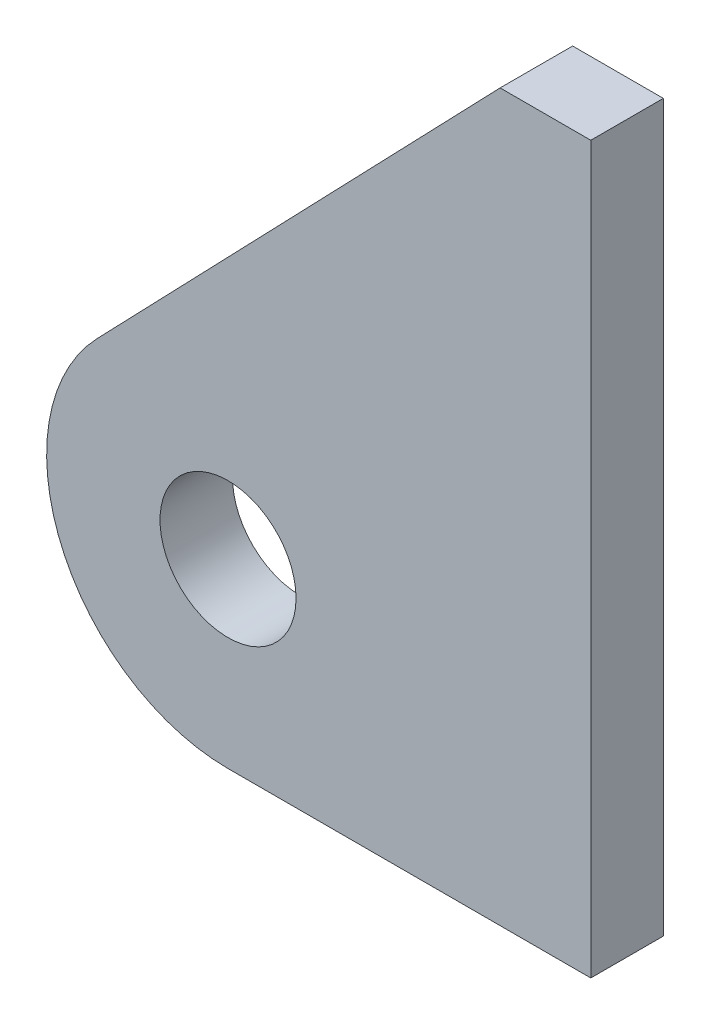
SolidWorks part; units mm, degrees
material "Q235B"
ref_plane "Front Plane" through (0, 0, 0) normal (0, 0, 1) x (1, 0, 0)
ref_plane "Top Plane" through (0, 0, 0) normal (0, 1, 0) x (1, 0, 0)
ref_plane "Right Plane" through (0, 0, 0) normal (1, 0, 0) x (0, 0, -1)
sketch "Sketch1" plane through (0, 0, 0) normal (0, 0, 1) x (1, 0, 0)
  line L0 (0, 0) -> (0, 80)
  line L1 (0, 80) -> (-10, 80)
  line L2 (-10, 80) -> (-54.4083, 33.8708)
  line L3 (-40, 0) -> (0, 0)
  arc A0 (-54.4083, 33.8708) -> (-40, 0) centre (-40, 20) ccw
  circle A1 centre (-40, 20) radius 7.5
  dimension "D1" = 40
  dimension "D4" = 20
  dimension "D5" = 15
  dimension "D2" = 80
  dimension "D3" = 10
extrude "Boss-Extrude1" add sketch "Sketch1" along normal mid plane 8
